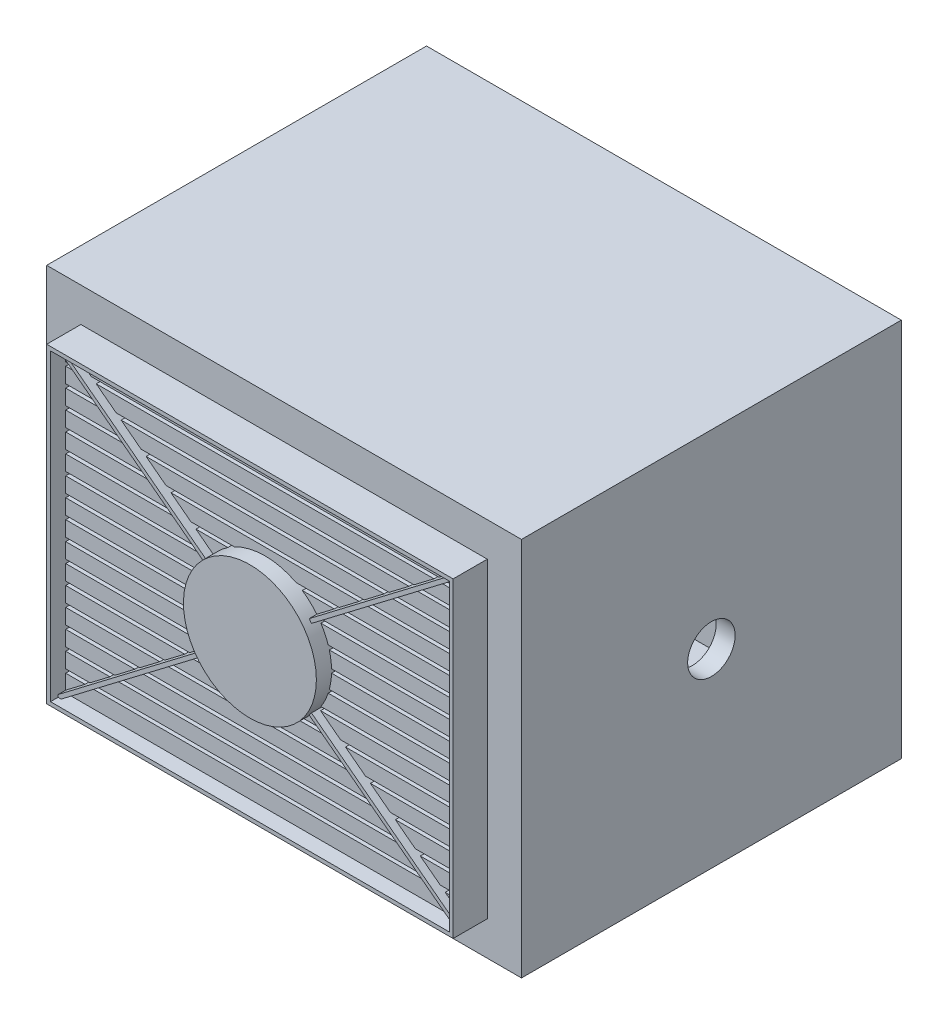
from build123d import *

# Parameters (mm, degrees)
SKETCH1_W               = 200
SKETCH1_H               = 200
BOSS_EXTRUDE1_DEPTH     = 125
SKETCH2_W               = 210
SKETCH2_H               = 160
BOSS_EXTRUDE2_DEPTH     = 10
SKETCH8_W               = 210
SKETCH8_H               = 2
CUT_EXTRUDE_THIN5_DEPTH = 2
LPATTERN1_COUNT         = 8
LPATTERN1_PITCH         = 10
LPATTERN1_COL_COUNT     = 8
LPATTERN1_COL_PITCH     = 10
SKETCH11_R              = 35
BOSS_EXTRUDE9_DEPTH     = 18
EXTRUDE_THIN2_DEPTH     = 14
EXTRUDE_THIN3_DEPTH     = 14
SKETCH14_W              = 214
SKETCH14_H              = 164
SKETCH14_W_2            = 210
SKETCH14_H_2            = 160
BOSS_EXTRUDE10_DEPTH    = 18
CUT_EXTRUDE1_START      = -10
SKETCH15_W              = 180
SKETCH15_H              = 180
CUT_EXTRUDE1_DEPTH      = 230
SKETCH16_R              = 12.5
CUT_EXTRUDE2_DEPTH      = 83


with BuildPart() as part:
    # Sketch1 → Boss-Extrude1 (new, symmetric)
    with BuildSketch(Plane(origin=(0, 0, 0), x_dir=(0, 0, -1), z_dir=(1, 0, 0))):
        Rectangle(SKETCH1_W, SKETCH1_H)
    extrude(amount=BOSS_EXTRUDE1_DEPTH, both=True)

    # Sketch2 → Boss-Extrude2 (add)
    with BuildSketch(Plane.XY.offset(100)):
        Rectangle(SKETCH2_W, SKETCH2_H)
    extrude(amount=BOSS_EXTRUDE2_DEPTH)

    # Sketch8 → Cut-Extrude-Thin5 (cut)
    with BuildSketch(Plane.XY.offset(110)):
        Rectangle(SKETCH8_W, SKETCH8_H)
    cut_extrude_thin5 = extrude(amount=-CUT_EXTRUDE_THIN5_DEPTH, mode=Mode.SUBTRACT)

    # LPattern1: Cut-Extrude-Thin5 ×8
    with Locations(*[(0, i * LPATTERN1_PITCH, 0) for i in range(1, LPATTERN1_COUNT)]):
        add(cut_extrude_thin5, mode=Mode.SUBTRACT)

    # LPattern1 col: Cut-Extrude-Thin5 ×8
    with Locations(*[(0, -i * LPATTERN1_COL_PITCH, 0) for i in range(1, LPATTERN1_COL_COUNT)]):
        add(cut_extrude_thin5, mode=Mode.SUBTRACT)

    # Sketch11 → Boss-Extrude9 (add)
    with BuildSketch(Plane.XY.offset(100)):
        with Locations(Location((0, 0, 0), (0, 0, 178.362754922))):
            Circle(SKETCH11_R)
    extrude(amount=BOSS_EXTRUDE9_DEPTH)

    # Sketch12 → Extrude-Thin2 (add)
    with BuildSketch(Plane.XY.offset(100)):
        Polygon((-105.606043215, 79.20456828), (104.393956785, -80.79543172), (105.606043215, -79.20456828), (-104.393956785, 80.79543172), align=None)
    extrude(amount=EXTRUDE_THIN2_DEPTH)

    # Sketch13 → Extrude-Thin3 (add)
    with BuildSketch(Plane.XY.offset(100)):
        Polygon((104.393956785, 80.79543172), (-105.606043215, -79.20456828), (-104.393956785, -80.79543172), (105.606043215, 79.20456828), align=None)
    extrude(amount=EXTRUDE_THIN3_DEPTH)

    # Sketch14 → Boss-Extrude10 (add)
    with BuildSketch(Plane.XY.offset(100)):
        Rectangle(SKETCH14_W, SKETCH14_H)
        Rectangle(SKETCH14_W_2, SKETCH14_H_2, mode=Mode.SUBTRACT)
    extrude(amount=BOSS_EXTRUDE10_DEPTH)

    # Sketch15 → Cut-Extrude1 (cut)
    with BuildSketch(Plane.ZY.offset(125).offset(CUT_EXTRUDE1_START)):
        Rectangle(SKETCH15_W, SKETCH15_H)
    extrude(amount=-CUT_EXTRUDE1_DEPTH, mode=Mode.SUBTRACT)

    # Sketch16 → Cut-Extrude2 (cut)
    with BuildSketch(Plane(origin=(125, 0, 0), x_dir=(0, 0, -1), z_dir=(1, 0, 0))):
        with Locations(Location((0, 0, 0), (0, 0, 90))):
            Circle(SKETCH16_R)
    extrude(amount=-CUT_EXTRUDE2_DEPTH, mode=Mode.SUBTRACT)


solid = part.part
